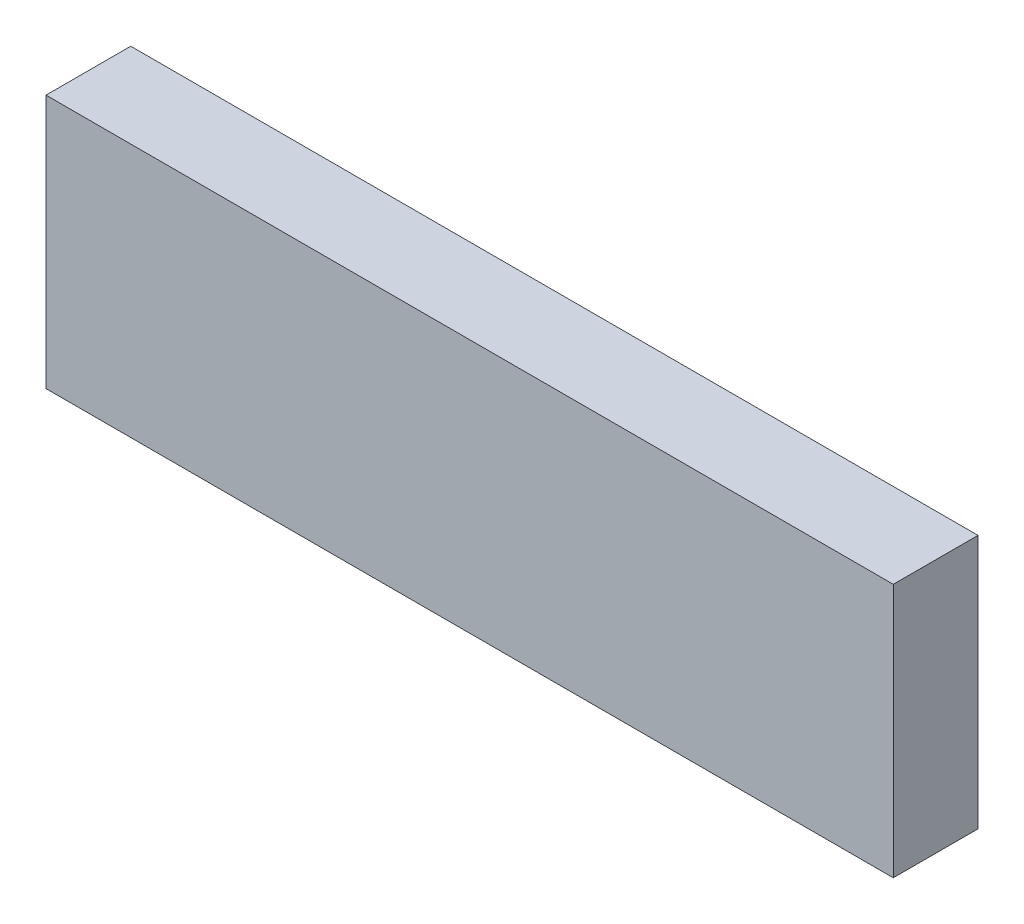
SolidWorks part; units mm, degrees
material "Q235B"
ref_plane "Front Plane" through (0, 0, 0) normal (0, 0, 1) x (1, 0, 0)
ref_plane "Top Plane" through (0, 0, 0) normal (0, 1, 0) x (1, 0, 0)
ref_plane "Right Plane" through (0, 0, 0) normal (1, 0, 0) x (0, 0, -1)
sketch "Sketch1" plane through (0, 0, 0) normal (0, 0, 1) x (1, 0, 0)
  line L1 (0, 0) -> (200, 0)
  line L2 (0, 0) -> (0, 60)
  line L3 (0, 60) -> (200, 60)
  line L4 (200, 0) -> (200, 60)
  dimension "D1" = 200
  dimension "D2" = 60
extrude "Boss-Extrude1" add sketch "Sketch1" along normal blind 20
